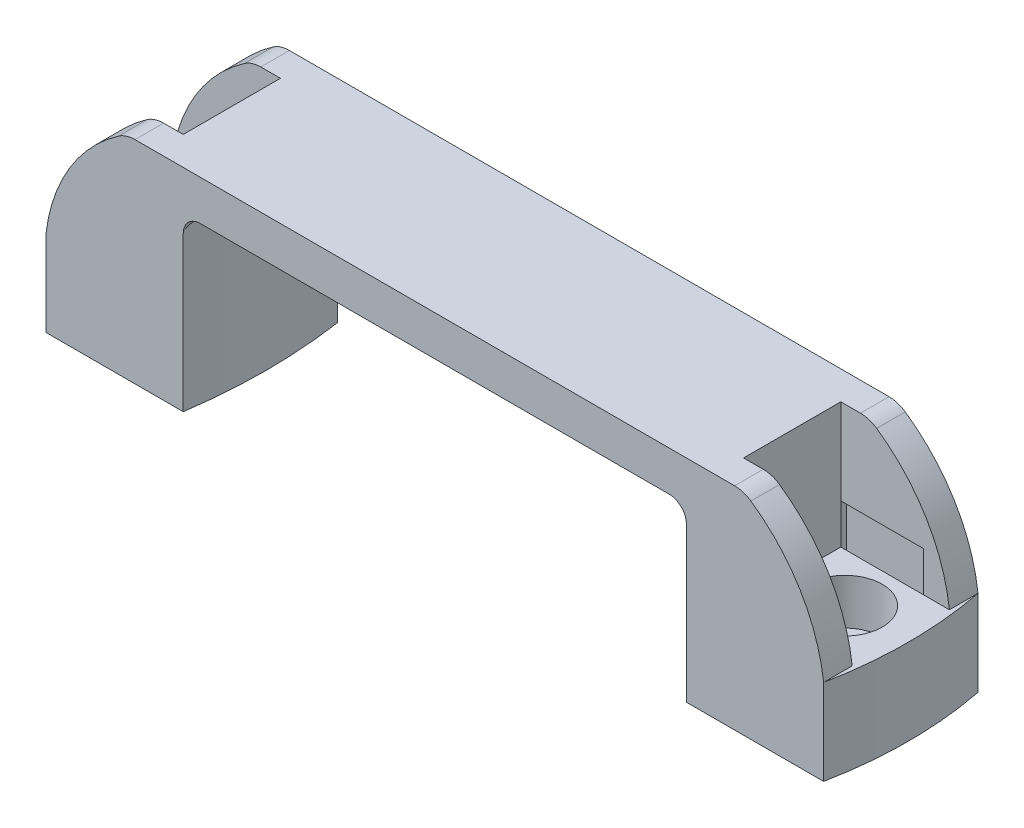
SolidWorks part; units mm, degrees
ref_plane "前视基准面" through (0, 0, 0) normal (0, 0, 1) x (1, 0, 0)
ref_plane "上视基准面" through (0, 0, 0) normal (0, 1, 0) x (1, 0, 0)
ref_plane "右视基准面" through (0, 0, 0) normal (1, 0, 0) x (0, 0, -1)
other "Configuration Table"
sketch "草图1" plane through (0, 0, 0) normal (0, 0, 1) x (1, 0, 0)
  line L0 (0, 0) -> (0, 54.6494) construction
  line L1 (-44, 0) -> (-68, 0)
  line L2 (-68, 0) -> (-68, 15)
  line L3 (-52.4386, 37) -> (52.4386, 37)
  line L4 (-44, 0) -> (-44, 27)
  line L5 (-41, 30) -> (41, 30)
  line L6 (-55.2839, 36.1114) -> (-54, 37) construction
  line L7 (-52.4386, 37) -> (-54, 37)
  line L8 (55.2839, 36.1114) -> (54, 37) construction
  line L9 (52.4386, 37) -> (54, 37)
  line L10 (44, 0) -> (44, 27)
  line L11 (68, 0) -> (68, 15)
  line L12 (44, 0) -> (68, 0)
  arc A0 (-68, 15) -> (-55.2839, 36.1114) centre (-38.2116, 11.4429) cw
  arc A1 (-52.4386, 37) -> (-55.2839, 36.1114) centre (-52.4386, 32) ccw
  arc A2 (-41, 30) -> (-44, 27) centre (-41, 27) ccw
  arc A3 (41, 30) -> (44, 27) centre (41, 27) cw
  arc A4 (52.4386, 37) -> (55.2839, 36.1114) centre (52.4386, 32) cw
  arc A5 (68, 15) -> (55.2839, 36.1114) centre (38.2116, 11.4429) ccw
  point P25 (0, 30)
  point P26 (0, 37)
  dimension "D1" = 30
  dimension "D4" = 5
  dimension "D8" = 3
  dimension "D2" = 68
  dimension "D3" = 7
  dimension "D5" = 37
  dimension "D6" = 15
  dimension "D7" = 44
  dimension "D9" = 54
extrude "凸台-拉伸1" add sketch "草图1" along normal mid plane 27 contours L11 A5 A4 L3 A1 A0 L2 L1 L4 A2 L5 A3 L10 L12
sketch "草图2" plane through (0, 0, 0) normal (0, -1, 0) x (1, 0, 0)
  line L0 (-56, 13.5) -> (-56, -13.5) construction
  line L1 (-44, 13.5) -> (-68, 13.5) construction
  line L2 (-44, -13.5) -> (-68, -13.5) construction
  line L3 (0, 0) -> (0, 13.5) construction
  line L4 (-44, 13.5) -> (-44, -13.5)
  line L5 (-41, 13.5) -> (41, 13.5) construction
  line L6 (56, 13.5) -> (56, -13.5) construction
  line L7 (44, 13.5) -> (44, -13.5)
  arc A0 (-44, -13.5) -> (-44, 13.5) centre (-134.625, 0) ccw
  arc A1 (44, -13.5) -> (44, 13.5) centre (134.625, 0) cw
  dimension "D2" = 90.625
extrude "凸台-拉伸2" add sketch "草图2" against normal up to surface (30 mm away) up to face at (0, 30, 0)
sketch "草图4" plane through (0, 0, 0) normal (0, -1, 0) x (1, 0, 0)
  line L1 (0, 0) -> (-69.3271, 0) construction
  line L2 (-68, 13.5) -> (-68, -13.5)
  line L3 (68, 13.5) -> (68, -13.5)
  arc A0 (68, -13.5) -> (68, 13.5) centre (0, 0) ccw
  arc A1 (-68, 13.5) -> (-68, -13.5) centre (0, 0) ccw
  dimension "D1" = 138.6542
extrude "凸台-拉伸3" add sketch "草图4" against normal up to vertex (15 mm away)
sketch "草图5" plane through (0, 0, 0) normal (0, 0, 1) x (1, 0, 0)
  line L0 (-68, 15) -> (-49, 15)
  line L1 (-49, 15) -> (-49, 37)
  line L2 (-52.4386, 37) -> (52.4386, 37) construction
  line L3 (0, 0) -> (0, 37) construction
  line L4 (-52.4386, 37) -> (-49, 37)
  line L5 (52.4386, 37) -> (49, 37)
  line L6 (49, 15) -> (49, 37)
  line L7 (68, 15) -> (49, 15)
  arc A0 (-52.4386, 37) -> (-55.2839, 36.1114) centre (-52.4386, 32) ccw construction
  arc A1 (-55.2839, 36.1114) -> (-68, 15) centre (-38.2116, 11.4429) ccw construction
  arc A2 (-52.4386, 37) -> (-55.2839, 36.1114) centre (-52.4386, 32) ccw
  arc A3 (-55.2839, 36.1114) -> (-68, 15) centre (-38.2116, 11.4429) ccw
  arc A4 (55.2839, 36.1114) -> (68, 15) centre (38.2116, 11.4429) cw
  arc A5 (52.4386, 37) -> (55.2839, 36.1114) centre (52.4386, 32) cw
  dimension "D1" = 49
extrude "切除-拉伸1" cut sketch "草图5" against normal mid plane 17 contours A2 A3 L0 L1 L4 | A5 L5 L6 L7 A4
sketch "草图6" plane through (0, 0, 0) normal (0, -1, 0) x (1, 0, 0)
  line L0 (0, 0) -> (-69.3271, 0) construction
  line L1 (-63.5, 11) -> (-47.5, 11)
  line L2 (-63.5, 11) -> (-63.5, 8.5)
  line L3 (-63.5, 8.5) -> (-47.5, 8.5)
  line L4 (-47.5, 11) -> (-47.5, 8.5)
  line L5 (0, 0) -> (0, 13.5) construction
  line L6 (-41, 13.5) -> (41, 13.5) construction
  line L7 (47.5, 11) -> (47.5, 8.5)
  line L8 (63.5, 8.5) -> (47.5, 8.5)
  line L9 (63.5, 11) -> (63.5, 8.5)
  line L10 (63.5, 11) -> (47.5, 11)
  line L11 (63.5, -11) -> (47.5, -11)
  line L12 (63.5, -11) -> (63.5, -8.5)
  line L13 (63.5, -8.5) -> (47.5, -8.5)
  line L14 (47.5, -11) -> (47.5, -8.5)
  line L15 (-63.5, -8.5) -> (-47.5, -8.5)
  line L16 (-63.5, -11) -> (-63.5, -8.5)
  line L17 (-47.5, -11) -> (-47.5, -8.5)
  line L18 (-63.5, -11) -> (-47.5, -11)
  arc A0 (-68, 13.5) -> (-68, -13.5) centre (0, 0) ccw construction
  dimension "D1" = 8.5
  dimension "D2" = 11
  dimension "D3" = 47.5
  dimension "D4" = 63.5
extrude "切除-拉伸2" cut sketch "草图6" against normal blind 22
sketch "草图7" plane through (0, 15, 0) normal (0, 1, 0) x (1, 0, 0)
  circle A0 centre (-58.25, 0) radius 6.5
  circle A1 centre (58.25, 0) radius 6.5
  dimension "D1" = 13
  dimension "D2" = 13
  dimension "D3" = 58.25
  dimension "D4" = 116.5
extrude "切除-拉伸3" cut sketch "草图7" against normal blind 8
sketch "草图8" plane through (0, 7, 0) normal (0, 1, 0) x (1, 0, 0)
  circle A0 centre (58.25, 0) radius 4.1
  circle A1 centre (-58.25, 0) radius 4.1
  dimension "D1" = 8.2
  dimension "D2" = 8.2
extrude "切除-拉伸4" cut sketch "草图8" against normal up to next
